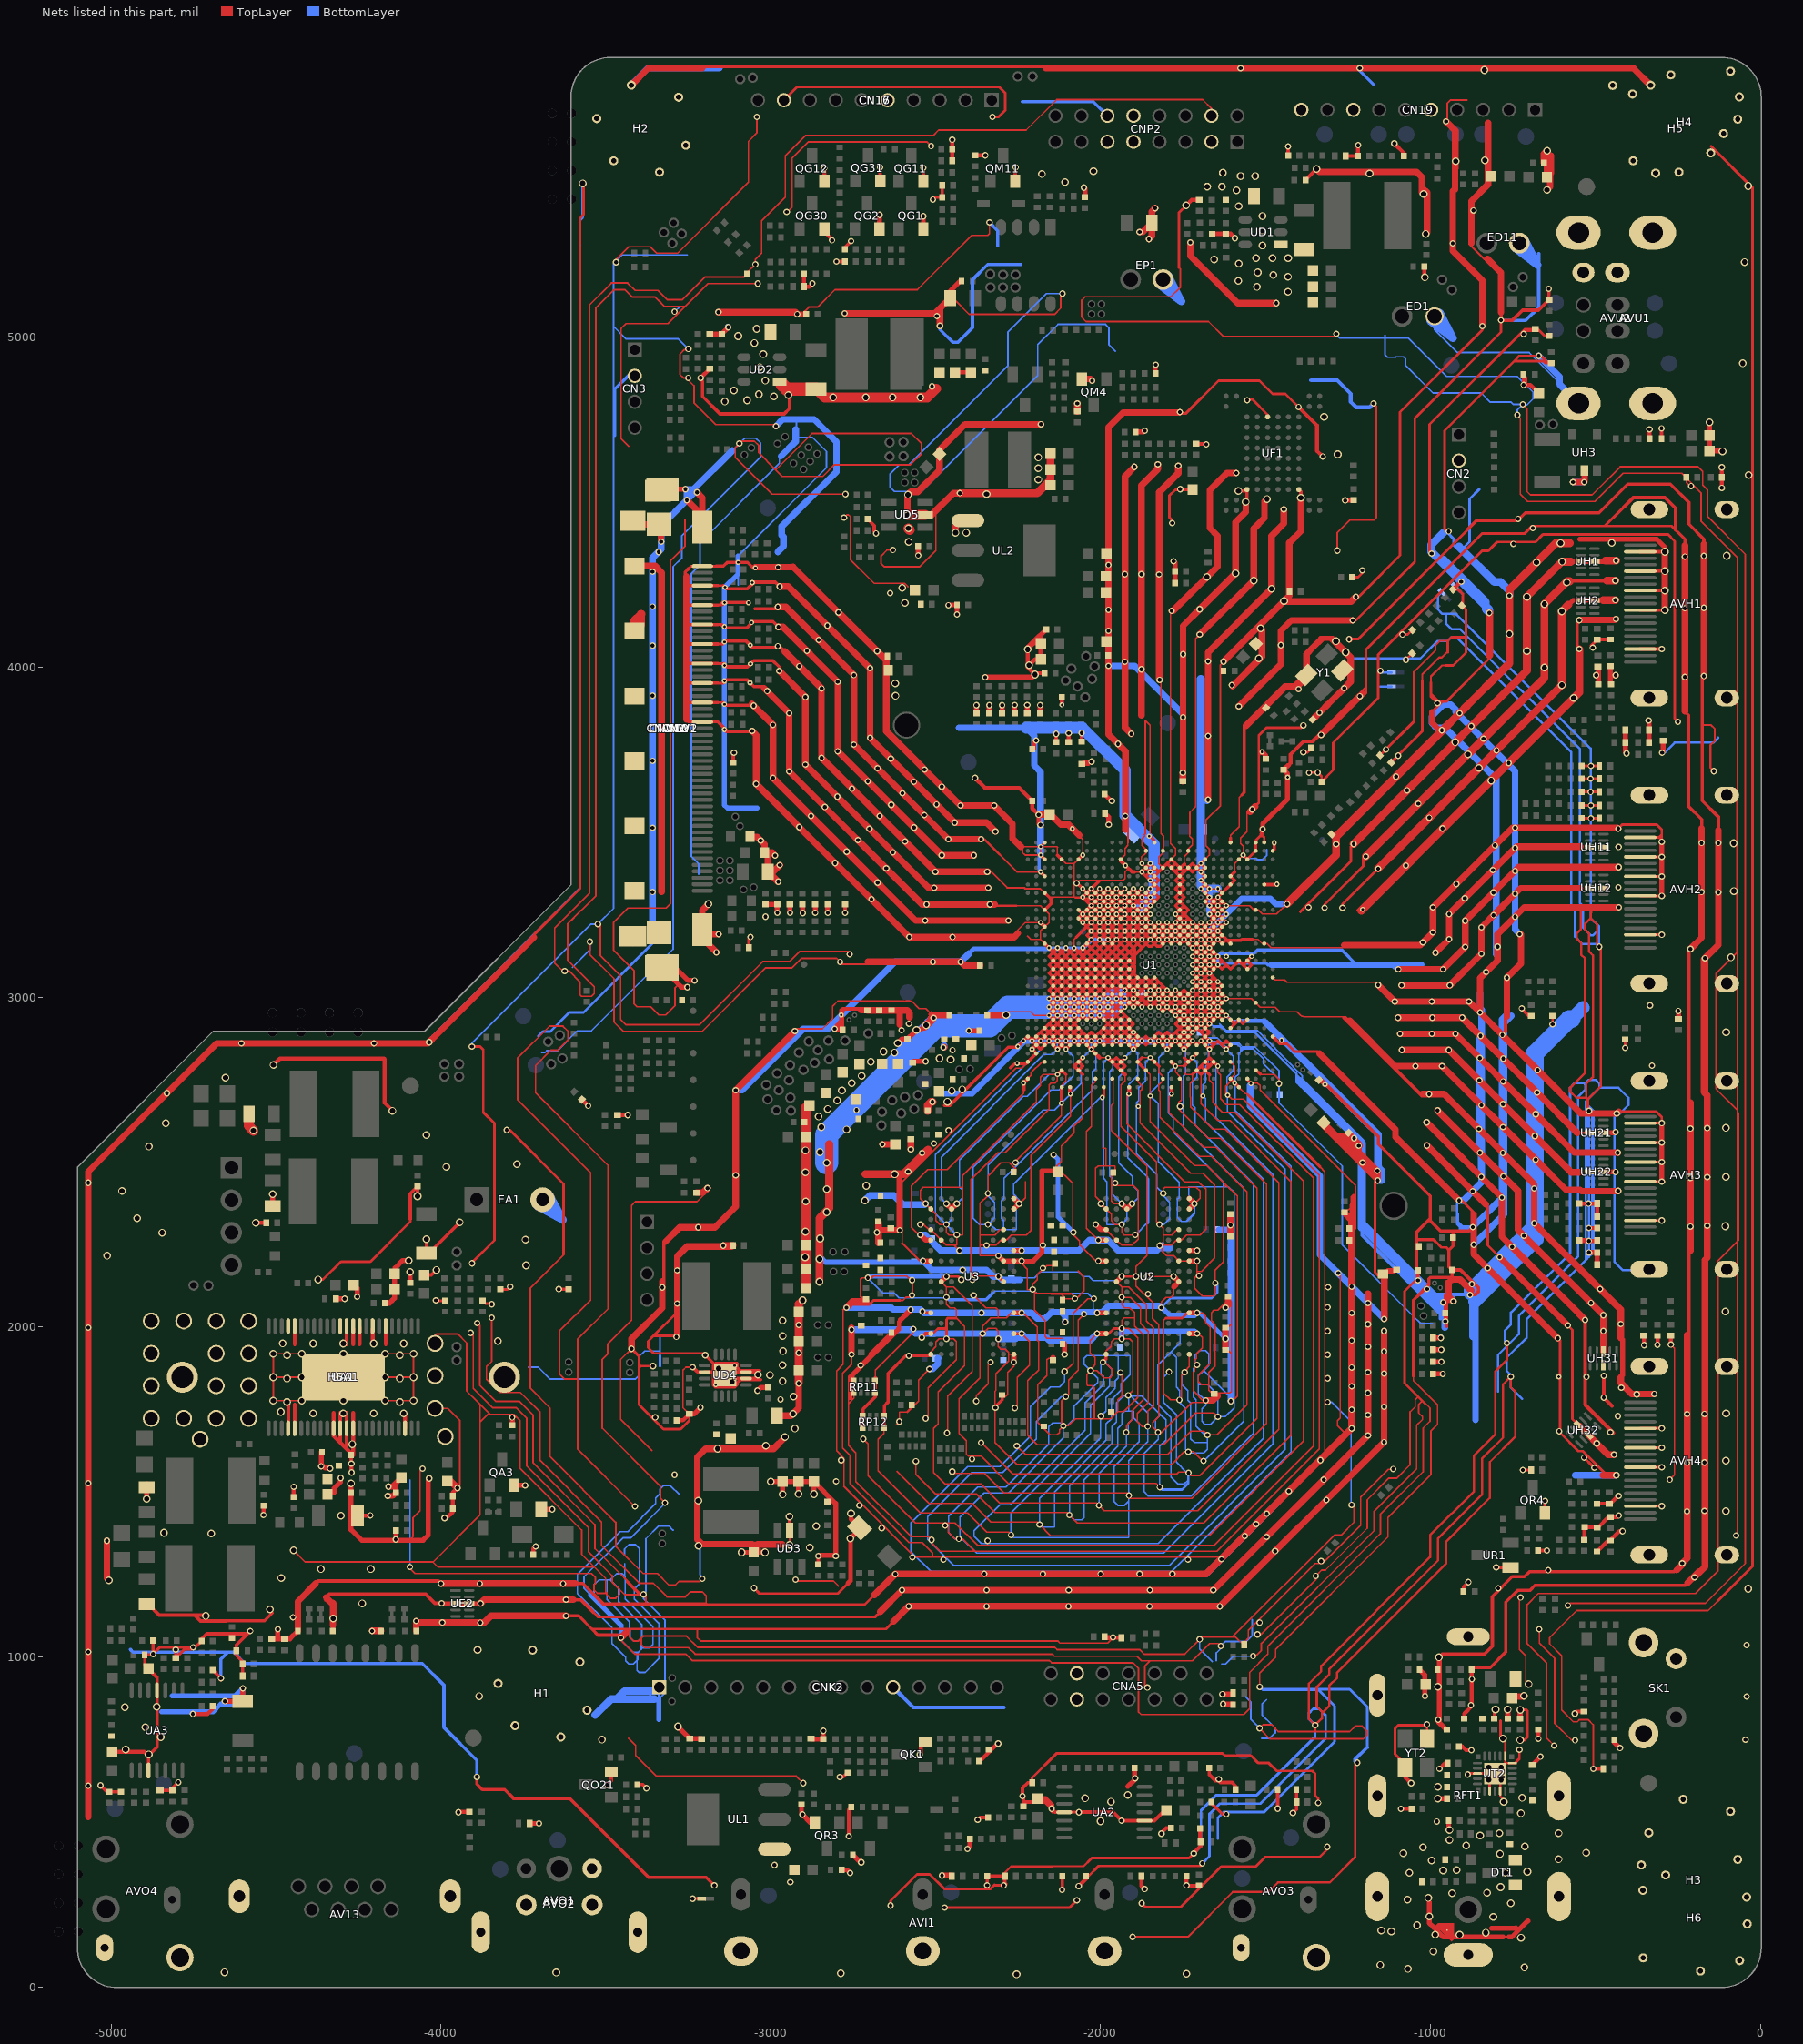
[diagram p0: the nets of this part, all layers, seen from the top]
# Altium PCB MISC86290.PcbDoc (part 16 of 31)
Units mil, origin at the board's own origin, x right, y up, seen from the top; angles counter-clockwise.
Board outline 5104.71 x 5851.49 mil, 2 copper layers (TopLayer, BottomLayer), stack 61.855 mil thick; 1026 components, 667 nets, 4280 pads, 2294 vias.

## Via types
v1: diameter 19.68, hole 11.81, TopLayer to BottomLayer, tented both sides, 1189 vias
v2: diameter 19.68/19.68 (per signal layer), hole 11.81, TopLayer to BottomLayer, tented both sides, 366 vias
v3: diameter 15.75, hole 7.87, TopLayer to BottomLayer, tented both sides, 348 vias
v4: diameter 23.62, hole 15.75, TopLayer to BottomLayer, tented both sides, 309 vias
v5: diameter 15.75/15.75 (per signal layer), hole 7.87, TopLayer to BottomLayer, tented both sides, 59 vias
v6: diameter 24/24 (per signal layer), hole 16, TopLayer to BottomLayer, tented both sides, 23 vias

## Nets (pads, with @x,y where several pads share a name; then routed paths per layer and width w, separated by ;. In a path a pad name is that pad's centre, name@x,y a point inside that pad or via, vN(x,y) a via of type N, cw(c..) or ccw(c..) an arc to the next point about the centre after c; other vN are vias at no path point) (continued)
GND: (continued)
  TopLayer w8: v4(-4372,2144) -4357.47,2144 -4303.22,2198.25 -4213.97,2198.25 -4093,2319.22 -4093,2326.45 ; v1(-4015,2081) -4013.73,2079.73 CA38.1@-3987,2079.73 ; v1(-3906.34,2849.93) -3881.23,2849.93 -3871.8,2840.5 -3871.8,2650.99 -3838.4,2617.59 -3838.4,2262.6 v1@-3906,2195 ; v1(-3906,2193) v1@-3906,2195 ; v1@-3900.5,2200.5 v1@-3906,2195 ; RA11.1@-3874,2079.73 -3865.27,2071 -3848,2071 v1(-3846,2069) ; CA39.1@-3820.35,2114.29 -3798.08,2114.29 v1(-3790.35,2122.03) ; v1(-3801,2597) -3791.08,2597 -3628.15,2434.07 -3628.15,2220.35 ; -3717.44,3180.84 -3717.44,3190.16 -3579.11,3328.49 -3579.11,5278.5 ; -3579.11,5283.17 -3579.11,5361.46 -3568,5372.57 -3568,5464.75 v4(-3570.25,5467) ; -3564.25,1106.25 -3542.5,1084.5 -3431,1084.5 -3222.5,1084.5 -2650.91,1084.5 -2627.95,1107.45 ; -3537.67,1134.83 -3524.34,1121.5 -2683.2,1121.5 -2668.1,1136.6 ; v1@-3422.5,1938.67 v1(-3422.5,1934) -3399,1910.5 -3399,1877.5 ; -3399,1885.5 -3395,1881.5 ; v1(-3357.5,1881.5) -3395,1881.5 ; v1@-3290,1972.84 -3355.8,1972.84 ; -3284,2049.5 -3284,2044.65 -3355.8,1972.84 ; -3256,3841.75 -3248.46,3834.21 CNW3.25@-3207.67,3834.21 -3159.77,3834.21 -3151.07,3825.51 ; -3255.49,4129.49 -3147.26,4129.49 v3(-3140.74,4122.97) ; -3254.38,4011.38 CNW3.16@-3207.67,4011.38 -3164.5,4011.38 ; -3253.43,4070.43 CNW3.13@-3207.67,4070.43 -3169,4070.43 ; -3250,3893.27 CNW3.22@-3207.67,3893.27 -3174.5,3893.27 ; -3250,3952.32 CNW3.19@-3207.67,3952.32 -3169,3952.32 ; -3250,4188.54 CNW3.7@-3207.67,4188.54 ; -3250,4247.6 v3@-3143.85,4247.6 ; -3249,4299.57 -3241.92,4306.65 CNW3.1@-3207.67,4306.65 -3143.59,4306.65 ; CD34.1@-3247.25,1736.27 -3247.25,1716.75 -3273.5,1690.5 -3325.5,1690.5 -3399,1764 -3399,1877.5 ; v1(-3237.25,267) RI116.JP_1K@-3210.25,267 ; -3156.43,4070.43 -3169,4070.43 ; -3154.7,4188.54 CNW3.7@-3207.67,4188.54 ; v3@-3144.1,4247.6 v3(-3139,4242.5) ; v3@-3143.52,3893.27 -3174.5,3893.27 ; v3@-3143.22,3952.32 -3169,3952.32 ; v3@-3142.63,4011.38 -3164.5,4011.38 ; v3(-3140.74,3887.58) -3146.42,3893.27 -3174.5,3893.27 ; v3(-3140.74,3958.87) -3147.29,3952.32 -3169,3952.32 ; v3(-3140.74,4005.42) -3146.69,4011.38 -3164.5,4011.38 ; v3(-3140.74,4076.72) -3147.02,4070.43 -3169,4070.43 ; v3(-3140.5,4195.5) -3147.46,4188.54 CNW3.7@-3207.67,4188.54 ; UD4.EPAD@-3138.01,1853.69 -3147.85,1863.53 -3170.05,1885.73 v1(-3199.03,1914.71) -3204.48,1920.16 -3355.3,1920.16 -3372.34,1937.2 -3372.34,1956.3 -3355.8,1972.84 ; v1(-3051,1208.5) -3034.68,1192.18 ; -3036.06,1192.18 -3034.68,1192.18 ; -3000.5,1192.18 -3034.68,1192.18 ; CN16.9@-2960.59,5719.46 -2919.94,5760.11 -2308.61,5760.11 -2290,5741.5 -2290,5688 -2309.5,5668.5 v1(-2328,5668.5) ; -2766,1223 -2796.82,1192.18 -3034.68,1192.18 ; v1(-2637,246) -2637,261 -2557,341 -2518,341 -2474,297 -2333.73,297 -2322,308.73 -2320.35,307.09 v1(-2294,307.09) ; v1(-2473.25,240) -2094.5,240 v1(-2072.5,262) ; DI2.A@-2290.73,340 DI2.A@-2288.27,340 ; RO57.1@-2207.96,618.5 -2207.96,632.77 ; -2207.96,633.04 -2133.16,707.84 -1676.84,707.84 ; v1(-2148.66,539.86) -2148.66,539.66 -2148.66,531.66 -2146,529 -2138,529 UA2.4@-2110.55,529 v1(-2066,529) ; CI3.1@-2044.54,334.99 -2037.01,334.99 -2006,366 -1698.84,366 v1@-1692,372.84 ; -2039,378 -2027,390 -1732,390 v1(-1718,404) ; v2(-1876,253) -1865,242 -1757,242 -1635,364 -1530.54,364 -1501.54,393 -1336.78,393 -1313,416.78 v2(-1313,424) ; v1(-1783,4437) -1783,4445.75 -1792.25,4455 -1792.25,4519.58 -1773.64,4538.19 CF3.1@-1721.5,4538.19 ; -1762.25,5211.58 -1762.25,5378.75 v4(-1741,5400) ; v1@-1751.36,4769.11 -1742.87,4769.11 -1642.99,4868.99 ; -1729.22,707.82 -1688,707.82 ; v3(-1721.77,3021.26) -1708.98,3008.46 v3(-1696.18,2995.67) U1.L9@-1683.39,2982.87 v3(-1670.59,2970.08) U1.K8@-1657.8,2957.28 v3(-1645,2944.49) U1.J7@-1632.2,2931.69 v3(-1619.41,2944.49) ; CF1.1@-1711,4677.73 CF1.1@-1710.27,4677 ; v1@-1681,4677 v1(-1680,4676) ; -1676.82,707.82 -1688,707.82 ; U1.K7@-1632.2,2957.28 v3(-1619.41,2944.49) ; v5(-1619.41,2842.13) U1.F6@-1606.61,2854.92 ; -1615,4868.99 -1642.99,4868.99 ; U1.J6@-1606.61,2931.69 v3(-1619.41,2944.49) ; v3(-1568.23,3430.71) U1.AH4@-1555.43,3417.91 U1.AJ3@-1529.84,3443.5 -1529.84,3475.27 -1511.29,3493.82 v1@-1511.29,3503.11 ; U1.J4@-1556.42,2931.69 U1.J4@-1555.43,2931.69 ; v1(-1555.95,4809.94) -1553.89,4812 -1540.1,4812 ; U1.B4@-1555.43,2752.56 -1555.43,2749.19 v3@-1544.32,2738.08 ; v1@-1547,4812 -1540.1,4812 ; -1531.92,3577.92 -1520.79,3589.05 -1520.79,3681.5 ; -1511.29,3491.86 -1504.25,3484.82 U1.AK2@-1504.25,3469.09 ; v3(-1510.98,3743.7) -1520.79,3733.89 -1520.79,3681.5 ; UF1.C5@-1493.75,4759.13 -1493.75,4765.65 -1540.1,4812 ; v2(-1459.22,2737.78) v2@-1457.99,2737.78 ; CT12.1@-1445.5,3689.27 CT12.1@-1439.94,3689.27 ; -1441,2858.95 -1436.01,2858.95 -1411.95,2834.89 -1390,2834.89 ; -1435.66,3694.19 -1426.66,3703.19 -1426.66,3735.84 ; -1433.5,3600.87 -1430,3604.37 -1430,3646.5 -1430.57,3646.5 ; -1426.66,3719 -1426.66,3735.84 ; v1(-1400.18,4789.18) -1440,4829 -1478.59,4829 -1518.59,4868.99 -1642.99,4868.99 ; v1(-1400,3934) -1400,3937.59 -1376.34,3961.26 Y1.4@-1376.34,3977.04 ; -1395.11,3258.42 -1241.56,3411.98 -1241.56,3456.5 v1(-1233.56,3464.5) ; -1385.72,3776.78 -1426.66,3735.84 ; v1(-1385.5,3742.5) -1372.95,3742.5 -1361.73,3753.72 CT13.1@-1361.73,3755.5 ; v1(-1385.5,3824) -1392.21,3817.29 -1496.7,3817.29 -1520.79,3793.2 -1520.79,3681.5 ; -1377.35,2834.89 -1390,2834.89 ; v1(-1370.3,3271.92) -1370.3,3283.23 ; v1(-1368.5,3680.5) -1368,3681 v1(-1342.5,3681) -1330.54,3669.04 LO1.2@-1330.54,3653 -1295,3688.54 -1295,3728 ; -1350.5,624.5 -1350.5,646.5 ; v1(-1340.5,557.5) -1340.5,570.5 -1350.5,580.5 -1350.5,646.5 ; -1336.52,2828.89 -1342.52,2834.89 -1390,2834.89 ; v1(-1321.19,3270.81) -1321.19,3280.02 -1204.56,3396.65 -1204.56,3426.65 v1@-1201.1,3430.1 ; -1313.54,2797.42 -1302,2785.88 -1293.51,2785.88 ; -1295,3715.32 -1295,3728 ; -1293.22,4199.11 -1232.66,4199.11 -1198.39,4233.39 ; -1269.61,4142.11 -1226.02,4142.11 -1047.75,4320.39 -1047.75,4754.68 -786.25,5016.18 v1(-786.25,5052) v1@-786.25,5060 ; v1(-1267.19,3270.81) -1267.19,3281.69 -1159.31,3389.57 v1(-1158.57,3389.57) ; v1(-1247,4085) -1246.89,4085.11 -1225,4085.11 ; v1@-1246,4085.11 -1225,4085.11 ; RU18.1@-1238.04,4273 -1219.58,4273 -1206.84,4285.75 v1(-1206.84,4294.01) ; v1(-1226.66,4213.38) -1218.4,4213.38 -1198.39,4233.39 ; -1226.38,3908.82 -1196.27,3938.93 ; -1220.76,3263.75 -1070.76,3413.75 ; -1202.92,3923.8 v1(-1214.36,3912.36) -1205.87,3912.36 -1196.27,3921.96 -1196.27,4053.07 -864.09,4385.25 -846.02,4403.32 -844.34,4405 -715.5,4405 -692.3,4428.2 v1@-683.8,4428.2 ; -1180.56,3442.55 -1201.1,3422 v1@-1201.1,3430.1 ; -1178.21,3456.21 -1178.21,3453 v1@-1201.1,3430.1 ; v1@-1168.75,2448.55 -1168.75,2436.5 ; v1(-1161.28,2473.58) -1168.75,2466.11 -1168.75,2436.5 ; RI115.1@-1153.17,3732.83 v1(-1135,3751) -1050.5,3835.5 -1050.5,3975.92 ; C201.1@-1138.85,2160.9 -1143.1,2160.9 -1153.5,2150.5 -1168.75,2165.75 -1168.75,2436.5 ; v1(-1098,3732) RI2.1@-1119.17,3710.83 -1119.17,3712.83 -1025.5,3806.5 -1025.5,3959 ; v1(-1085,4099) -1069.18,4099 CO51.1@-1055.4,4112.78 ; -1079,1848.5 -1079,1872.5 ; YT2.2@-1077.46,674.46 -1108.12,705.12 -1108.12,782.59 -1097.71,793 -1013,793 v1(-1011,795) -1010.54,794.54 YT2.4@-1010.54,751.31 ; v1(-1074.56,3398.64) -1064.1,3409.1 ; DO2.A@-1038.96,2167.5 -1038.96,2148.05 -1079,2108.02 -1079,1872.5 ; -1015.44,1766.2 -1079,1829.76 -1079,1872.5 ; v1@-1002.75,4349.75 v1@-1002.75,4350.25 ; -1002.75,4374.5 v1@-1002.75,4350.25 ; -998.84,3955 -998.84,3920.2 ; v1(-996.91,4345) -997.5,4345 v1@-1002.75,4350.25 ; -995.5,3864.77 -963.43,3896.84 ; -986.64,2261.02 -967.06,2241.43 -952.41,2241.43 -944.34,2233.37 ; v1(-979,3891) -998.84,3910.84 -998.84,3920.2 ; -956,4005.84 -931.21,4005.84 -893,4044.06 -893,4087 ; -947.84,4044.84 -947.84,4048 -947.84,4079.8 -936.8,4090.84 -896.84,4090.84 -893,4087 ; v1(-945,4412) -951.6,4412 -957.75,4418.15 -957.75,4717.4 -746.65,4928.5 ; RO53.1@-932.74,4235.43 -915.43,4235.43 -901.99,4221.99 -901.99,4190.01 RO54.1@-905.17,4186.83 -893,4174.66 -893,4087 ; v1(-913.55,2383.45) -905.07,2383.45 -875.59,2353.97 ; -875.59,2239.23 -875.59,2353.97 ; -863.59,2340 -863.59,2341.97 -875.59,2353.97 ; -859.49,4445 -1219.39,4085.11 -1225,4085.11 ; -843.25,5075.42 -843.25,5022.82 -1092.75,4773.32 -1092.75,4339.03 -1198.39,4233.39 ; -832.59,2371.78 -826.59,2365.78 -826.59,2247.53 v1(-790.53,2211.47) ; -822,4037.28 -822,4025.96 -951.12,3896.84 -963.43,3896.84 ; UT2.EPAD@-804.89,646.37 UT2.EPAD@-773.4,677.86 ; -787.53,807.21 -787.53,759.29 v4(-780.91,752.66) v4@-773.4,745.16 ; v1(-748.89,4374.16) v1@-754.74,4380 ; v4(-728.53,747.65) -715.28,747.65 -706.03,756.9 -706.03,836.67 ; v4@-728.39,839.29 v4(-728.03,839.65) -727.52,840.16 -709.53,840.16 ; v1(-720.5,1566.5) DR1.A@-695.23,1566.5 ; v1(-718,5010) -707.86,5020.14 -687.26,5020.14 DU2.A@-682.3,5025.1 ; v1(-690,4422) v1@-683.8,4428.2 ; v1@-673,4946 -672,4945 v1(-672,4944) ; -665.5,4428.2 v1@-683.8,4428.2 ; DF5.A@-637.32,5004.53 DF5.A@-641.25,5004.53 -654.53,5004.53 -675.1,5025.1 DU2.A@-682.3,5025.1 ; DU1.A@-634,4922.27 DU1.A@-643.84,4922.27 ; v1(-614.18,1965.82) -607.38,1959.02 -607.38,1679.38 -551.73,1623.73 -538.41,1623.73 -471.34,1556.66 -455,1556.66 ; v1(-584,2004.94) -570.38,1991.32 -570.38,1721.22 UH32.GND@-551.03,1701.87 ; CH17.1@-541.27,3541.99 -514.01,3541.99 DH15.A@-488.73,3542 ; CH14.2@-541.27,3581.01 v1(-514,3581) DH14.A@-488.73,3581 ; CH13.2@-541.27,3621.99 -515.01,3621.99 DH13.A@-488.73,3622 ; CH12.2@-541.27,3662.01 v1(-515.01,3662.01) DH12.A@-488.73,3662 ; CH11.2@-541.27,3701.01 v1(-514.01,3701.01) DH11.A@-488.73,3701 ; v1(-534.53,1604) v1@-510,1579.46 ; -447,4453 -471.8,4428.2 ; v1(-435.5,2647.5) -430.01,2653 -429.22,2653 -315.61,2653 -299,2636.39 v2(-299,2618) -299.11,2618.11 AVH3.2@-364.47,2618.11 ; v1(-431,3511) -419.4,3522.6 -313.6,3522.6 -299,3508 v1(-299,3471) -299,3476 -307.25,3484.25 ; v1(-410,2846) CH18.1@-410,2872.27 ; AVH4.17@-364.47,1456.69 v2@-299.06,1456.69 ; AVH4.11@-364.47,1574.8 v2@-299.06,1574.8 ; AVH4.8@-364.47,1633.86 v2@-299.06,1633.86 ; AVH4.5@-364.47,1692.91 v2@-299.06,1692.91 ; AVH3.17@-364.47,2322.84 v2@-299.06,2322.84 ; AVH3.5@-364.47,2559.06 -299.06,2559.06 v2(-299,2559) ; AVH2.17@-364.47,3188.98 v2@-296.05,3188.98 ; AVH2.11@-364.47,3307.09 v2@-296.05,3307.09 ; AVH2.8@-364.47,3366.14 v2@-296.05,3366.14 ; AVH2.5@-364.47,3425.2 v2@-296.05,3425.2 ; AVH2.2@-364.47,3484.25 -307.25,3484.25 ; v2@-299.06,2440.95 AVH3.11@-364.47,2440.95 v2@-296.05,2440.95 ; v2@-299.06,2500 AVH3.8@-364.47,2500 v2@-297,2500 ; -299,3492.51 -307.25,3484.25 ; v1(-250,3835) -260,3845 -260,4382.32 -280.88,4403.2 -658.8,4403.2 -682,4380 v1@-754.74,4380 ; -246.95,4406.05 -257.5,4416.59 -269.11,4428.2 -471.8,4428.2 ; -149.87,5579.72 -24.5,5454.35 -24.5,1274.13 -128.81,1169.81 ; AVH1.23@-103.22,4478.35 AVH1.23@-72.1,4478.35 ; -3399,1877.5 -3395,1881.5 ; -1688,707.82 -1631.32,707.82 -1623.75,700.25 -1544.26,700.25 -1522.01,678 -1490.21,678 -1466.42,654.2 -1358.2,654.2 -1350.5,646.5 ; -1295,3728 -1295,3770.9 -1159.27,3906.63 -1159.27,4037.74 -843.38,4353.63 -824.63,4353.63 -798.26,4380 v1@-754.74,4380 ; v1@-1002.75,4350.25 -1002.75,4736.04 -713.68,5025.1 DU2.A@-682.3,5025.1 ; -998.84,3920.2 -975.49,3896.84 -963.43,3896.84 ; -746.65,4928.5 -731.15,4944 v1(-672,4944) ; -746.65,4928.5 -658.24,4928.5 -652,4922.27 DU1.A@-643.84,4922.27 ; v1@-683.8,4428.2 -471.8,4428.2 ; v1(-672,4944) -665.57,4944 DU1.A@-643.84,4922.27
  TopLayer w9.8: -3248.46,3893.27 CNW3.22@-3207.67,3893.27 -3159.77,3893.27 ; -3248.46,3952.32 CNW3.19@-3207.67,3952.32 -3159.77,3952.32 ; -3248.46,4011.38 CNW3.16@-3207.67,4011.38 -3159.77,4011.38 ; -3248.46,4070.43 CNW3.13@-3207.67,4070.43 -3159.77,4070.43 ; -3248.46,4129.49 CNW3.10@-3207.67,4129.49 -3159.77,4129.49 ; -3248.46,4188.54 CNW3.7@-3207.67,4188.54 -3159.77,4188.54 ; -3248.46,4247.6 CNW3.4@-3207.67,4247.6 -3159.77,4247.6
  TopLayer w9.84: RP12.8@-2720.79,1694.49 RP12.7@-2720.79,1720.53 ; RP12.7@-2720.79,1737.8 RP12.7@-2720.79,1720.53 ; -2683.39,1847.03 -2683.39,1788.43 -2720.79,1751.03 RP12.7@-2720.79,1720.53 ; RP12.2@-2655.83,1694.49 -2655.83,1761.42 -2644.02,1773.23 -2644.02,1859.84 -2590.87,1912.99 v2(-2582.01,1912.99) -2517.05,1912.99 -2515.08,1914.96 U3.T1@-2515.08,1916.93 ; v2(-2540.67,2046.85) -2536.73,2042.91 U3.M1@-2515.08,2042.91 ; v2(-2310.35,2153.15) U3.J8@-2294.61,2137.4 ; U3.P9@-2263.11,1979.92 v2(-2239.49,1979.92) ; v2(-1993.43,1893.31) -1983.58,1903.15 U2.T1@-1983.58,1916.93